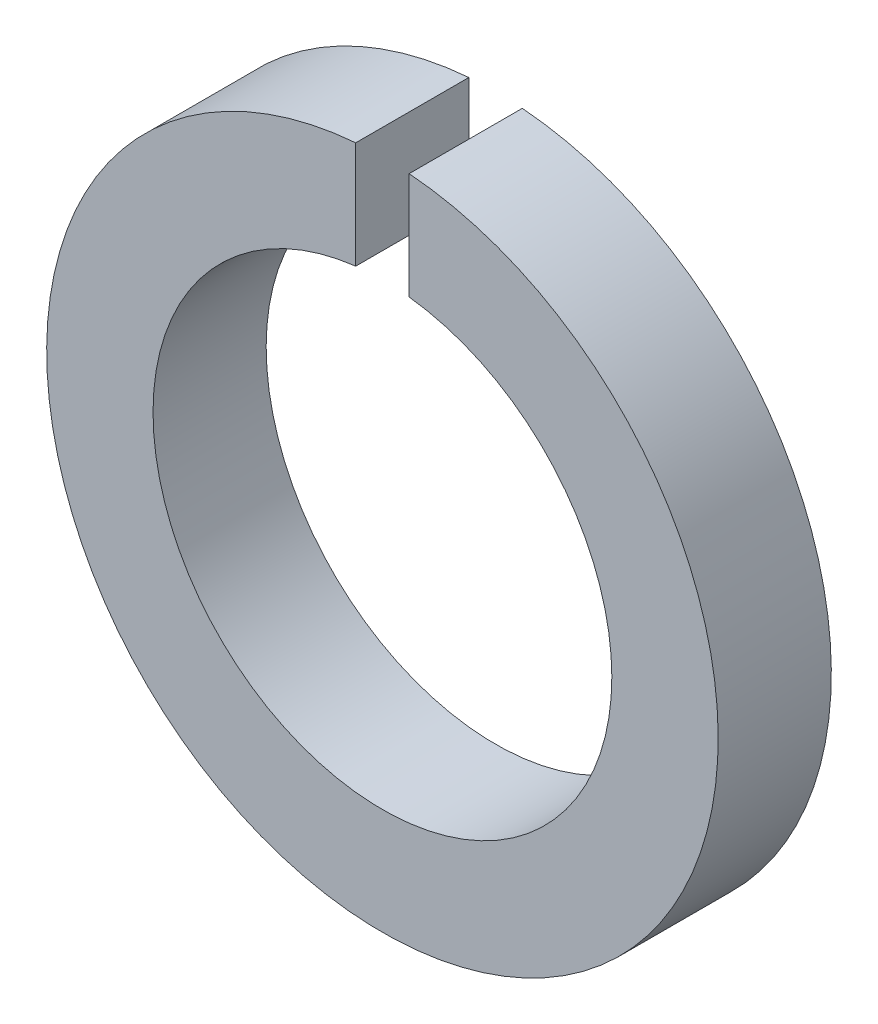
from build123d import *

# Parameters (mm, degrees)
EXTRUDE_1_DEPTH = 9


with BuildPart() as part:
    # 草图1 → 拉伸1 (new body)
    with BuildSketch(Plane.XY):
        with BuildLine():
            Line((-2.125, 26.625862048), (-2.125, 18.125862048))
            ThreePointArc((-2.125, 18.125862048), (0, -18.25), (2.125, 18.125862048))
            Line((2.125, 18.125862048), (2.125, 26.625862048))
            ThreePointArc((2.125, 26.625862048), (0, -26.710525169), (-2.125, 26.625862048))
        make_face()
    extrude(amount=EXTRUDE_1_DEPTH)


solid = part.part
